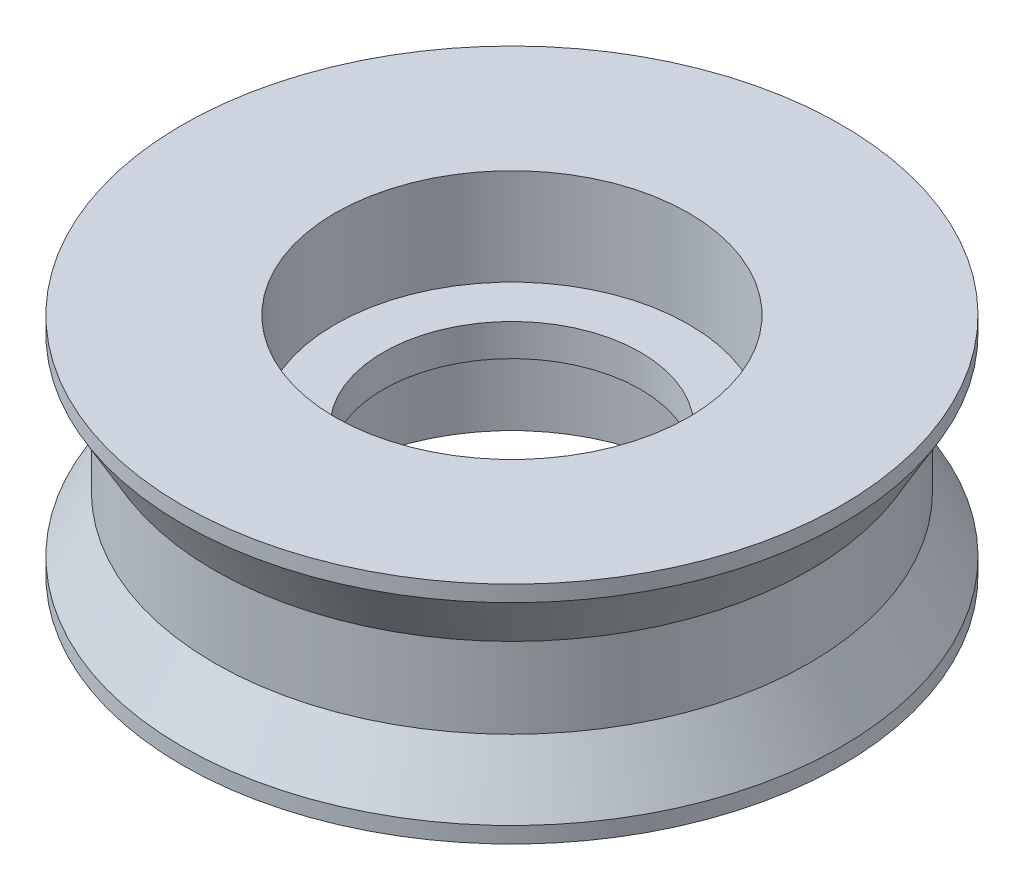
from build123d import *


with BuildPart() as part:
    # 草图1 → 旋转1 (revolve)
    with BuildSketch(Plane.XY, mode=Mode.PRIVATE) as revolve_1_sk:
        Polygon((20.5, -6), (18.5, -2.5), (18.5, 2.5), (20.5, 6), (20.5, 7), (11, 7), (11, 1), (8, 1), (8, -1), (11, -1), (11, -7), (20.5, -7), align=None)
    revolve(revolve_1_sk.sketch.rotate(Axis((0, 20.639192491, 0), (0, -1, 0)), 90), axis=Axis((0, 20.639192491, 0), (0, -1, 0)))


solid = part.part
